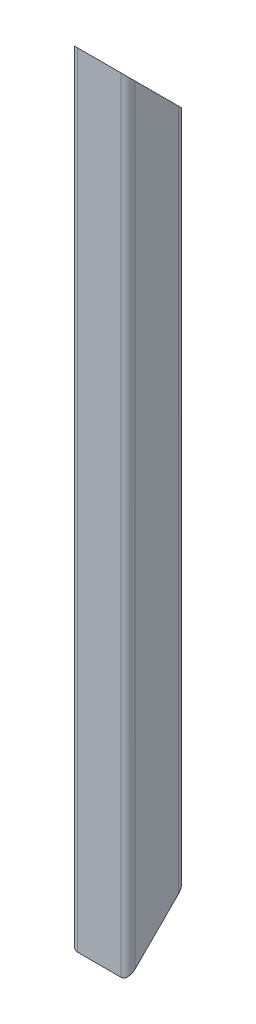
from build123d import *

# Parameters (mm, degrees)
EXTRUDE_1_DEPTH     = 680
CUT_EXTRUDE_1_DEPTH = 683.878423476


with BuildPart() as part:
    # 草图1 → 凸台-拉伸1 (new body)
    with BuildSketch(Plane(origin=(0, 0, 0), x_dir=(1, 0, 0), z_dir=(0, 1, 0))):
        with BuildLine():
            Line((-19, -12.278106509), (19, -12.278106509))
            ThreePointArc((19, -12.278106509), (23.242640687, -10.520747196), (25, -6.278106509))
            Line((25, -6.278106509), (25, 31.721893491))
            ThreePointArc((25, 31.721893491), (23.242640687, 35.964534178), (19, 37.721893491))
            Line((19, 37.721893491), (-19, 37.721893491))
            ThreePointArc((-19, 37.721893491), (-23.242640687, 35.964534178), (-25, 31.721893491))
            Line((-25, 31.721893491), (-25, -6.278106509))
            ThreePointArc((-25, -6.278106509), (-23.242640687, -10.520747196), (-19, -12.278106509))
        make_face()
        with BuildLine():
            Line((-19, -7.278106509), (19, -7.278106509))
            ThreePointArc((19, -7.278106509), (19.707106781, -6.98521329), (20, -6.278106509))
            Line((20, -6.278106509), (20, 31.721893491))
            ThreePointArc((20, 31.721893491), (19.707106781, 32.429000272), (19, 32.721893491))
            Line((19, 32.721893491), (-19, 32.721893491))
            ThreePointArc((-19, 32.721893491), (-19.707106781, 32.429000272), (-20, 31.721893491))
            Line((-20, 31.721893491), (-20, -6.278106509))
            ThreePointArc((-20, -6.278106509), (-19.707106781, -6.98521329), (-19, -7.278106509))
        make_face(mode=Mode.SUBTRACT)
    extrude(amount=EXTRUDE_1_DEPTH)

    # 草图2 → 切除-拉伸1 (cut, through all)
    with BuildSketch(Plane(origin=(25, 0, 0), x_dir=(0, 0, -1), z_dir=(1, 0, 0))):
        Polygon((-12.278106509, 680), (37.721893491, 680), (37.721893491, 630), align=None)
        Polygon((-12.278106509, 0), (37.721893491, 50), (37.721893491, 0), align=None)
    extrude(amount=-CUT_EXTRUDE_1_DEPTH, mode=Mode.SUBTRACT)


solid = part.part
